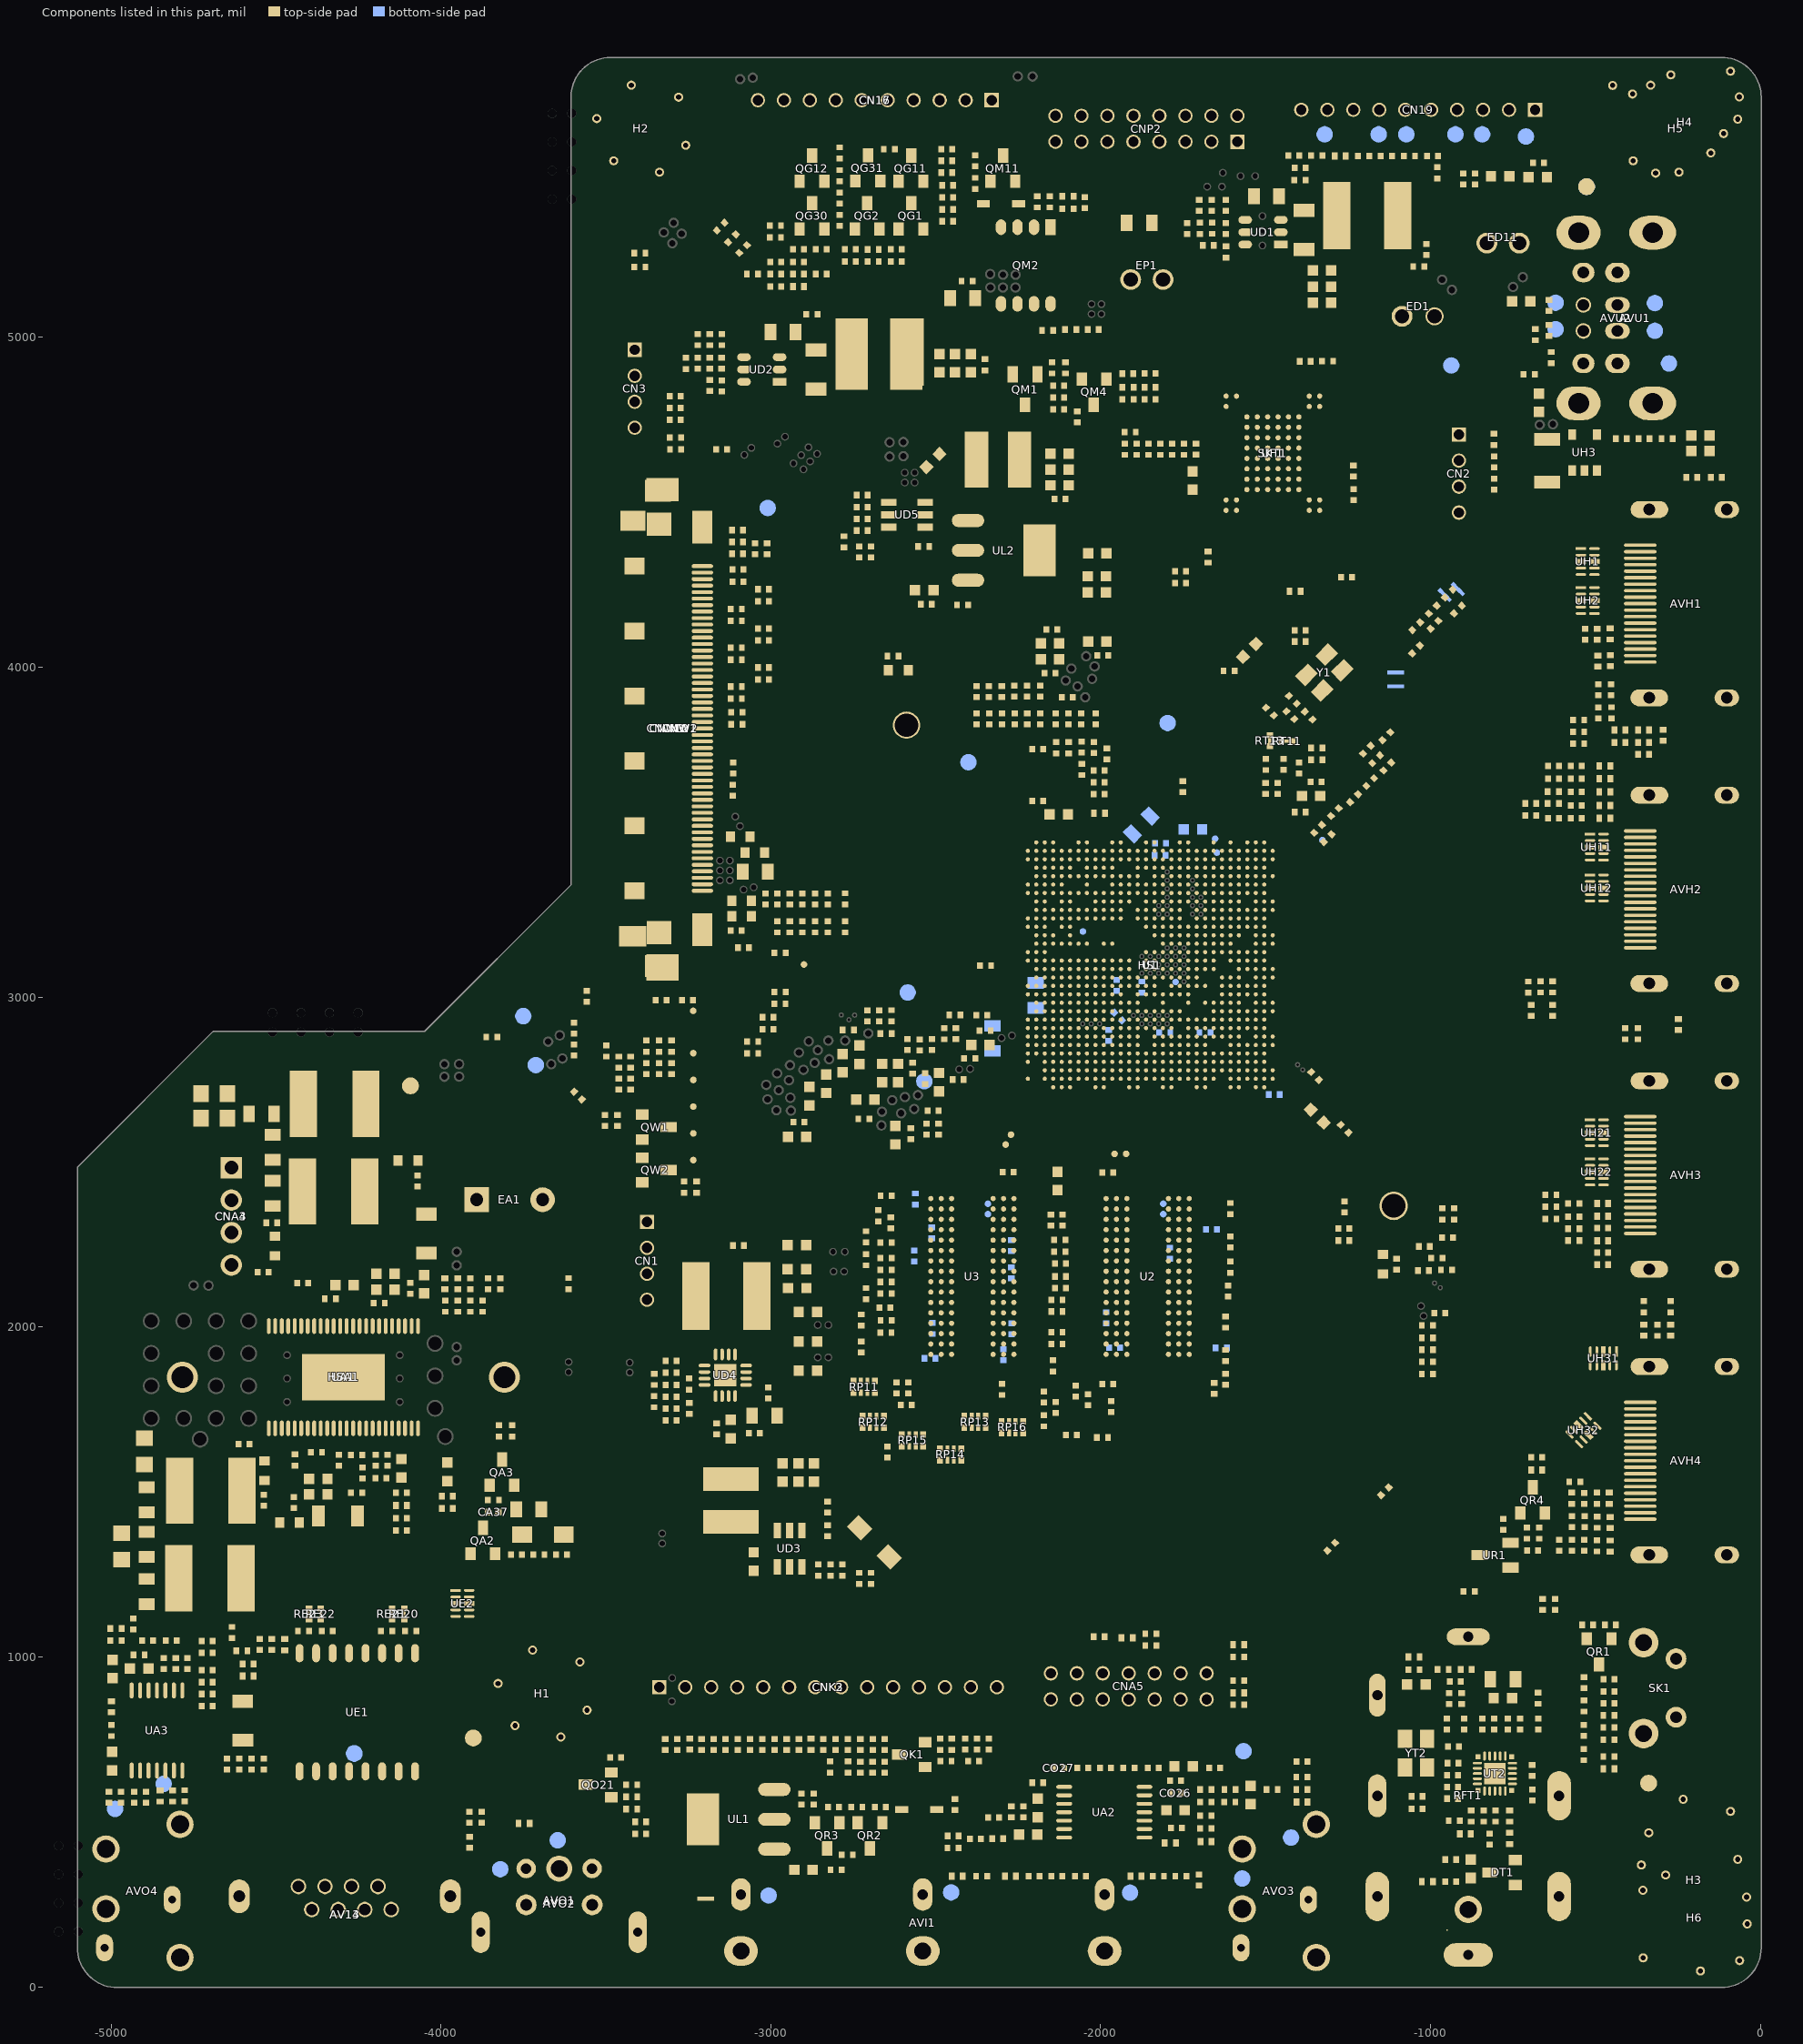
[diagram p0: the components of this part, seen from the top]
# Altium PCB MISC86290.PcbDoc (part 31 of 31)
Units mil, origin at the board's own origin, x right, y up, seen from the top; angles counter-clockwise.
Board outline 5104.71 x 5851.49 mil, 2 copper layers (TopLayer, BottomLayer), stack 61.855 mil thick; 1026 components, 667 nets, 4280 pads, 2294 vias.

## Silkscreen, mask and mechanical layers (free items; w line width, h text height) (continued)
附加说明:
  region: -5099.68,118.11 -5158.73,118.11 -5158.73,476.38 -5099.68,476.38 hole: -5129.2,286.04 -5140.4,297.24 -5129.2,308.44 -5118,297.24
  region: -3603.61,5370.08 -3662.67,5370.08 -3662.67,5728.35 -3603.61,5728.35 hole: -3633.14,5538.01 -3644.34,5549.21 -3633.14,5560.41 -3621.94,5549.21
  region: -4202,2952.76 -4202,2893.7 -4560.27,2893.7 -4560.27,2952.76 hole: -4369.93,2923.23 -4381.13,2912.03 -4392.33,2923.23 -4381.13,2934.43
  lines w5: 5582.82,5878.74 6712.82,5878.74 ; 5582.82,5986.08 6712.82,5986.08 ; 5582.82,6093.41 6712.82,6093.41 ; 5582.82,6200.74 6712.82,6200.74 ; 5582.82,6308.08 7013.32,6308.08 ; 5883.32,5771.41 5883.32,6415.41 ; 6712.82,5771.41 6712.82,6415.41 ; 5582.82,5771.41 5582.82,6415.41 7013.32,6415.41 7013.32,5771.41 5582.82,5771.41
  text "Template date:" at 3386.66,6343.42 h60
  text "Version cycle number" at 5604.66,6342.25 h60
  text "PCB designer" at 6160.16,6341.75 h60
  text "Customer" at 6823.16,6342.25 h60
  text "2018.03.20" at 3708.66,6339.92 h60
  text "Board utilization:" at 3386.16,6246.42 h60
  text "8X%" at 3708.66,6242.42 h60
  text "(Filled in for non-TV division projects)" at 3898.66,6242.42 h60
  text "PERSON_A__" at 6077.5,6240.5 h60
  text "XXXXXX" at 5624.16,6235.25 h60
  text "LLX" at 6119,6139.5 h60
  text "XXXXXX" at 5633.66,6129.25 h60
  text "MXZ" at 6119,6031.76 h60
  text "CO_B" at 6752.16,6024.92 h60
  text "XXXXXX" at 5633.66,6021.51 h60
  text "Special requirements; leave blank if none" at 1976.82,5845.76 h60
  text "The remark items below must be copied to the TopOverlay layer; one or two items may be remarked" at 2974.16,3264.92 h60
  text "Chip parts 3.5mm from PCB clamping edge; production requires special control" at 2269.16,3182.92 h60
  text "Height values and reference designators of solder-side chip parts over 2mm; leave blank if none" at 2267.22,2969.97 h60
  text "Easily damaged part reference designators; leave blank if none" at 2265.45,2823.81 h60
  text "New footprint reference designators; leave blank if none" at 2267.82,2616.76 h60
  text "Vacuum nozzle and press-pin positions reserved: enter Yes, otherwise No" at 2268.66,2413.92 h60
  text "X.XXXX.XXX Stencil Revision Explanation" at 1341.44,-406.05 h60
  text "X.XXXX.XXX Testing jig Revision Explanation" at 1340.94,-475.05 h60
  text "X.XXXX.XXX Wave-soldering jig Revision Explanation" at 1340.44,-543.05 h60
DrillDrawing:
  text ".Legend" at 1349.48,6463.64 h60